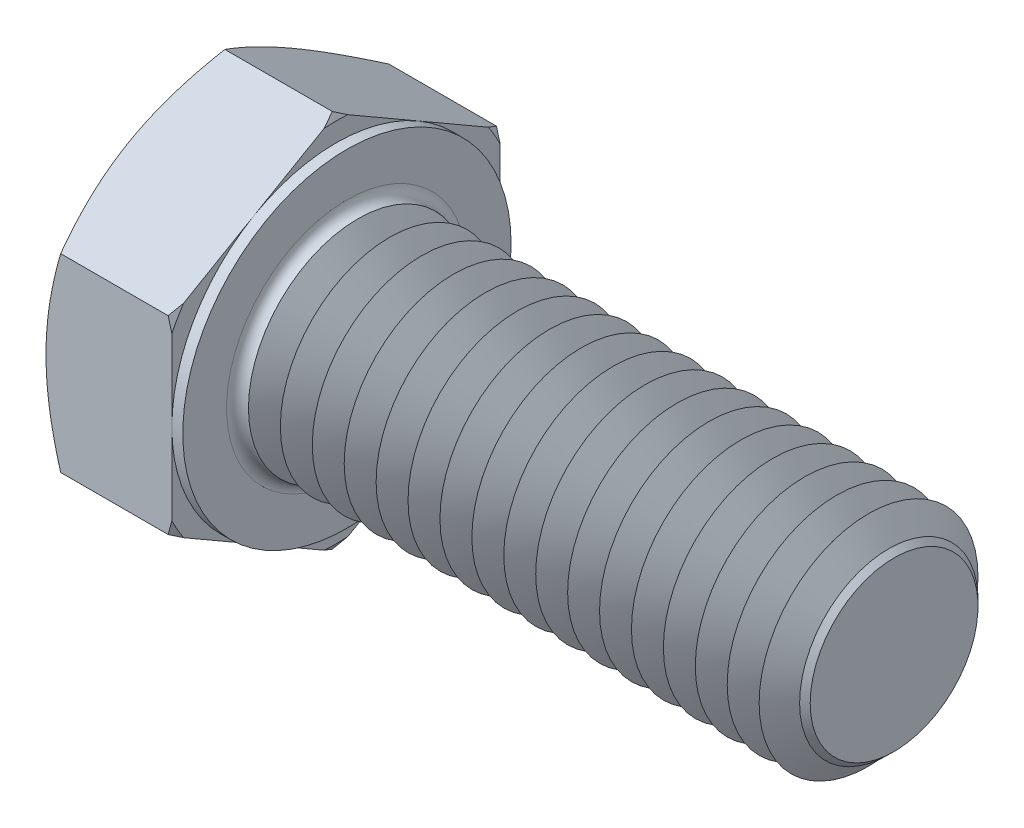
SolidWorks part; units mm, degrees
extrude "基体-拉伸" add sketch "草图1" along normal blind 7.5
sketch "草图1" plane through (0, 0, 0) normal (1, 0, 0) x (0, 0, -1)
  line L0 (9, 5.1962) -> (9, -5.1962)
  line L1 (-9, 5.1962) -> (-9, -5.1962)
  line L2 (9, -5.1962) -> (0, -10.3923)
  line L3 (0, -10.3923) -> (-9, -5.1962)
  line L4 (9, 5.1962) -> (0, 10.3923)
  line L5 (0, 10.3923) -> (-9, 5.1962)
revolve "切除-旋转1" cut sketch "草图3" angle 360 about L6
sketch "草图3" plane through (0, 0, 0) normal (0, 0, 1) x (1, 0, 0)
  line L0 (0, 9) -> (3.6906, 15.3923)
  line L1 (0, 10.3923) -> (0, 5.1962) construction
  line L2 (3.6906, 15.3923) -> (3.6906, 20.3923)
  line L3 (3.6906, 20.3923) -> (-10, 20.3923)
  line L4 (-10, 20.3923) -> (-10, 9)
  line L5 (-10, 9) -> (0, 9)
  line L6 (0, 0) -> (99.06, 0) construction
  line L7 (7.5, 10.3923) -> (0, 10.3923) construction
revolve "凸台-旋转1" add sketch "草图2" angle 360 about L7
sketch "草图2" plane through (0, 0, 0) normal (0, 0, 1) x (1, 0, 0)
  line L0 (0, 5.1962) -> (0, -5.1962) construction
  line L1 (0, 0) -> (37.5, 0)
  line L2 (0, 0) -> (0, 6)
  line L3 (0, 6) -> (37.5, 6)
  line L4 (37.5, 0) -> (37.5, 4.4845)
  line L5 (7.5, 10.3923) -> (7.5, 5.1962) construction
  line L7 (0, 0) -> (96.52, 0) construction
  line L8 (37.5, -4.4845) -> (90.335, -6) construction
  line L9 (0, -6) -> (90.335, -6) construction
  line L10 (9.25, 15.24) -> (9.25, -1.27) construction
  line L11 (7.5, 15.24) -> (7.5, -1.27) construction
  line L12 (7.5, 5.1962) -> (7.5, -5.1962) construction
  line L14 (37.5, 6) -> (37.5, 4.4845)
  dimension "l" = 30
  dimension "m" = 12
  dimension "Minor_dia" = 8.969
  dimension "p" = 1.75
  dimension "h" = 30
cosmetic thread "螺旋线1" parameters "Thread_length"=28.25, "Thread_minor"=8.969
material "5.6级"
ref_plane "前视" through (0, 0, 0) normal (0, 0, 1) x (1, 0, 0)
ref_plane "上视" through (0, 0, 0) normal (0, 1, 0) x (1, 0, 0)
ref_plane "右视" through (0, 0, 0) normal (1, 0, 0) x (0, 0, -1)
sketch "草图5" plane through (0, 0, 0) normal (0, 0, 1) x (1, 0, 0)
  line L0 (7.5, 9) -> (3.8094, 15.3923)
  line L1 (7.5, 10.3923) -> (7.5, 5.1962) construction
  line L2 (3.8094, 15.3923) -> (3.8094, 20.3923)
  line L3 (3.8094, 20.3923) -> (13.8094, 20.3923)
  line L4 (13.8094, 20.3923) -> (13.8094, 9)
  line L5 (13.8094, 9) -> (7.5, 9)
  line L7 (7.5, 10.3923) -> (0.8038, 10.3923) construction
  line L8 (0, 0) -> (99.06, 0) construction
  line L9 (0, 0) -> (99.06, 0) construction
revolve "切除-旋转2" cut sketch "草图5" angle 360 about L8
sketch "草图4" plane through (0, 0, 0) normal (0, 0, 1) x (1, 0, 0)
  line L1 (7.5, 10.3923) -> (7.5, 5.1962) construction
  line L2 (7.5, 9) -> (6.9, 9)
  line L3 (7.5, 9) -> (7.5, 20.3923)
  line L4 (7.5, 20.3923) -> (6.9, 20.3923)
  line L5 (0, 0) -> (95.25, 0) construction
  line L6 (0, 0) -> (96.52, 0) construction
  line L7 (6.9, 9) -> (6.9, 20.3923)
  line L8 (6.6962, 10.3923) -> (0.8038, 10.3923) construction
revolve "切除-旋转3" cut sketch "草图4" angle 360 about L5
chamfer "倒角" distance 1.4 angle 45 1 edges at (37.5, 0, 6)
fillet "圆角" radius 0.6 1 edges at (7.5, 0, -6)
sketch "草图6" plane through (0, 0, 0) normal (0, 0, 1) x (1, 0, 0)
  line L0 (8.975, -4.4845) -> (8.1, -6)
  line L1 (8.975, -4.4845) -> (9.8499, -6)
  line L2 (9.8499, -6) -> (9.8499, -7.5)
  line L3 (-3.175, 0) -> (5.1513, 0) construction
  line L5 (9.8499, -7.5) -> (8.1, -7.5)
  line L6 (8.1, -7.5) -> (8.1, -6)
  arc A0 (8.1, -6) -> (7.5, -6.6) centre (8.1, -6.6) ccw construction
revolve "切除-旋转4" cut sketch "草图6" angle 360 about L3
pattern_linear "阵列(线性)1" count 17 spacing 1.75 along (1, 0, 0) of "切除-旋转4"
equation "\"D3@草图1\" = \"s@草图1\" / 2"
equation "\"D4@草图1\" = \"D3@草图1\""
equation "\"D5@草图1\" = \"D4@草图1\""
equation "\"D1@草图3\" = \"s@草图1\" / 2"
equation "\"D1@草图5\" = \"s@草图1\" / 2"
equation "\"Head_ch_ang@草图5\" = \"Head_ch_ang@草图3\""
equation "\"D1@草图4\" = \"s@草图1\""
equation "\"Diameter@草图6\" = \"m@草图2\""
equation "\"Overcut@草图6\" = \"m@草图2\" * 1.25"
equation "\"Minor_dia@草图2\" = \"m@草图2\"-\"p@草图2\" * 1.732"
equation "\"Thread_minor@螺旋线1\" = \"Minor_dia@草图2\""
equation "\"Thread_minor@草图6\" = \"Minor_dia@草图2\""
equation "\"D1@倒角\" = \"p@草图2\"*0.8"
equation "\"Thread_length@螺旋线1\" = \"l@草图2\" - \"p@草图2\""
equation "\"Num_threads@阵列(线性)1\" = \"l@草图2\" / \"p@草图2\""
